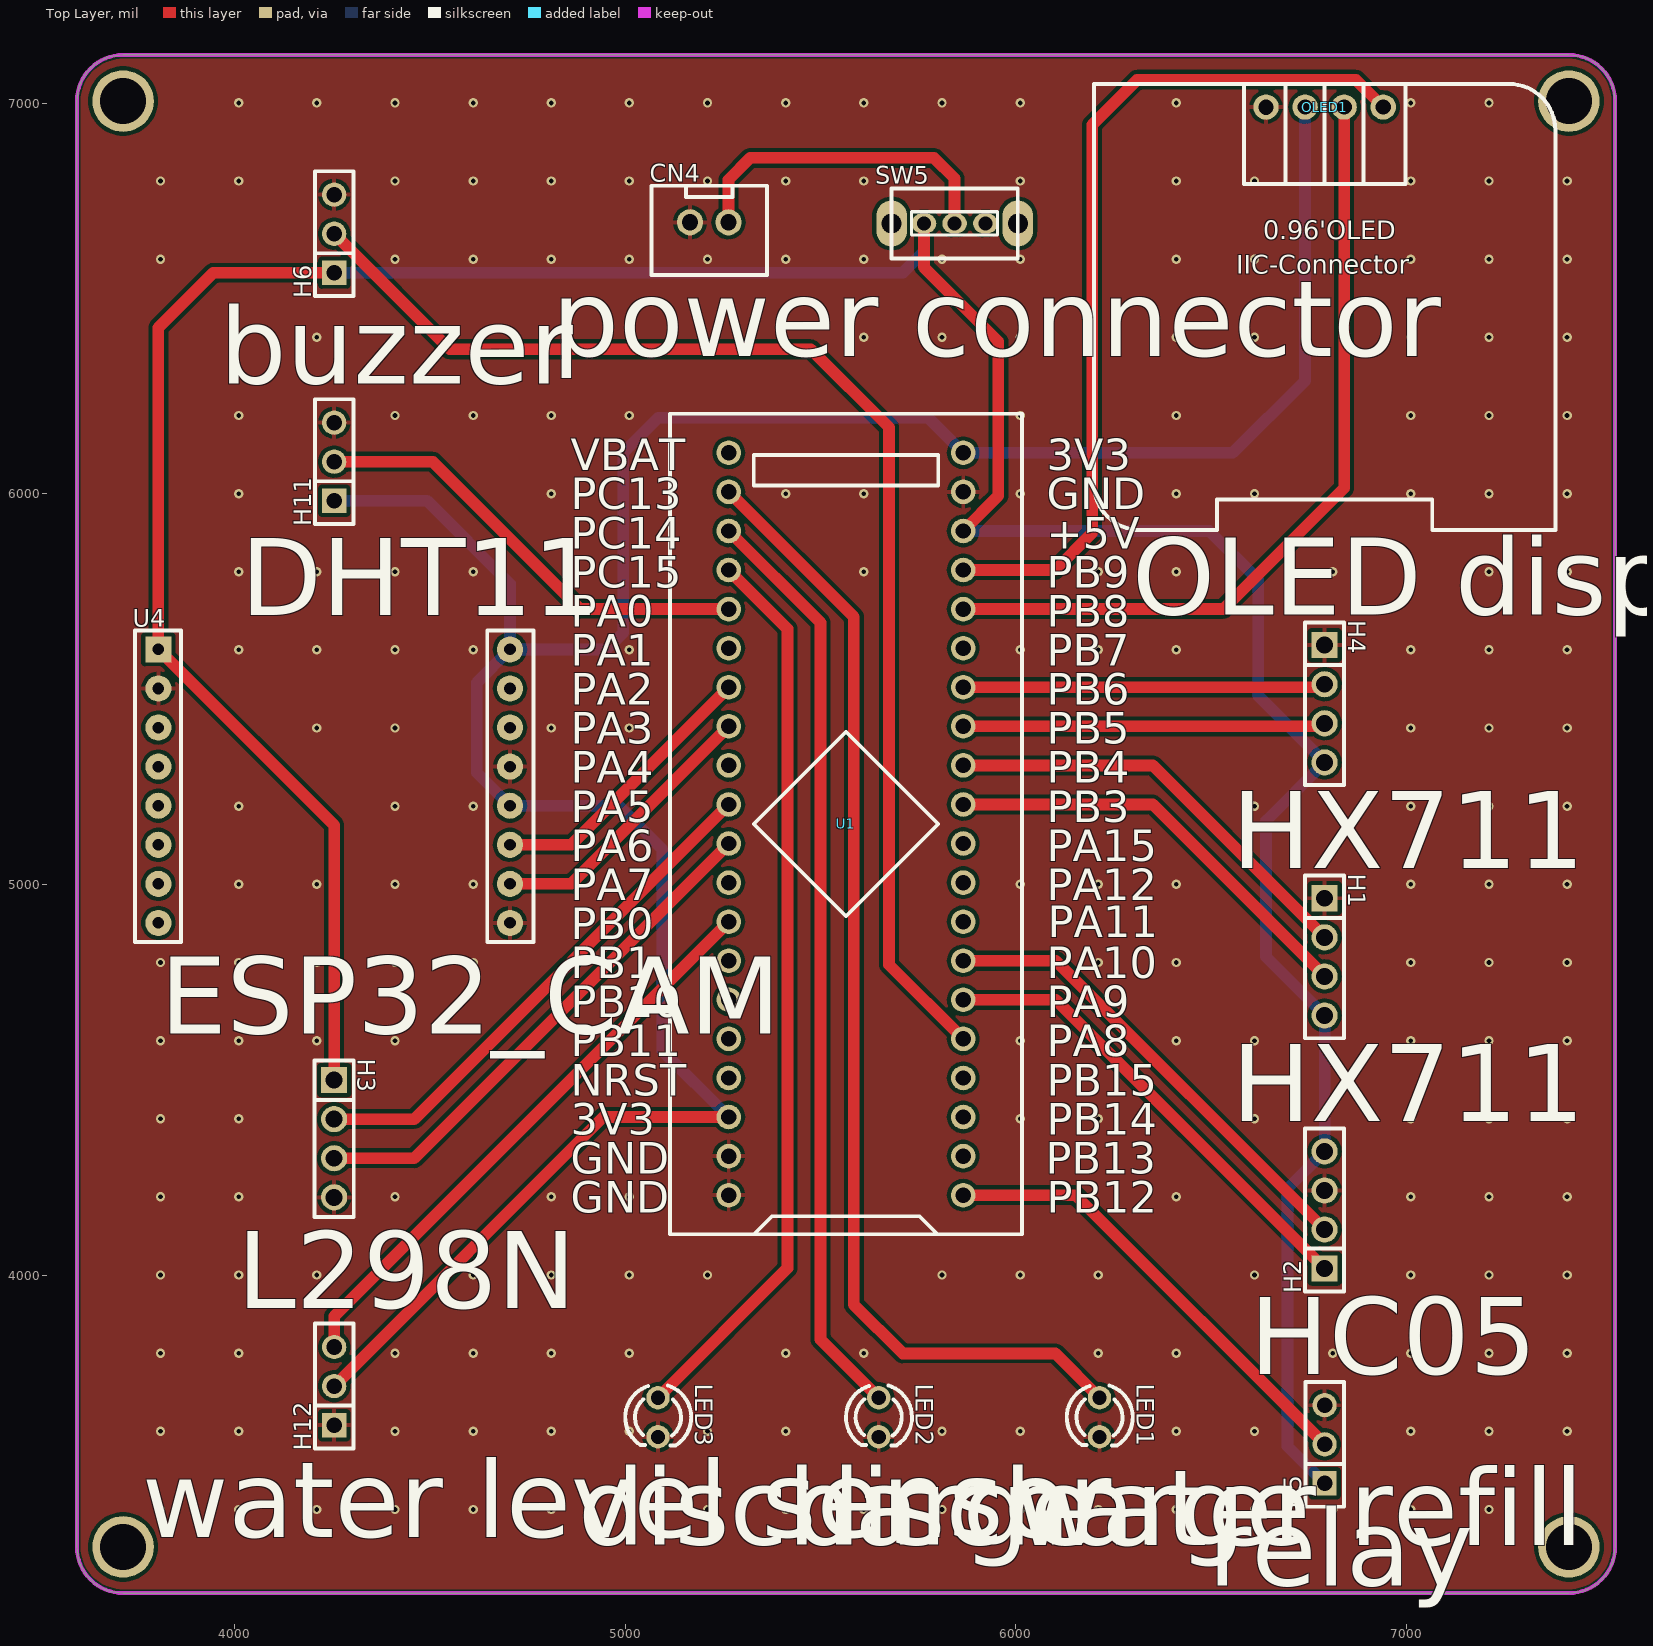
[diagram p0: Top Layer view]
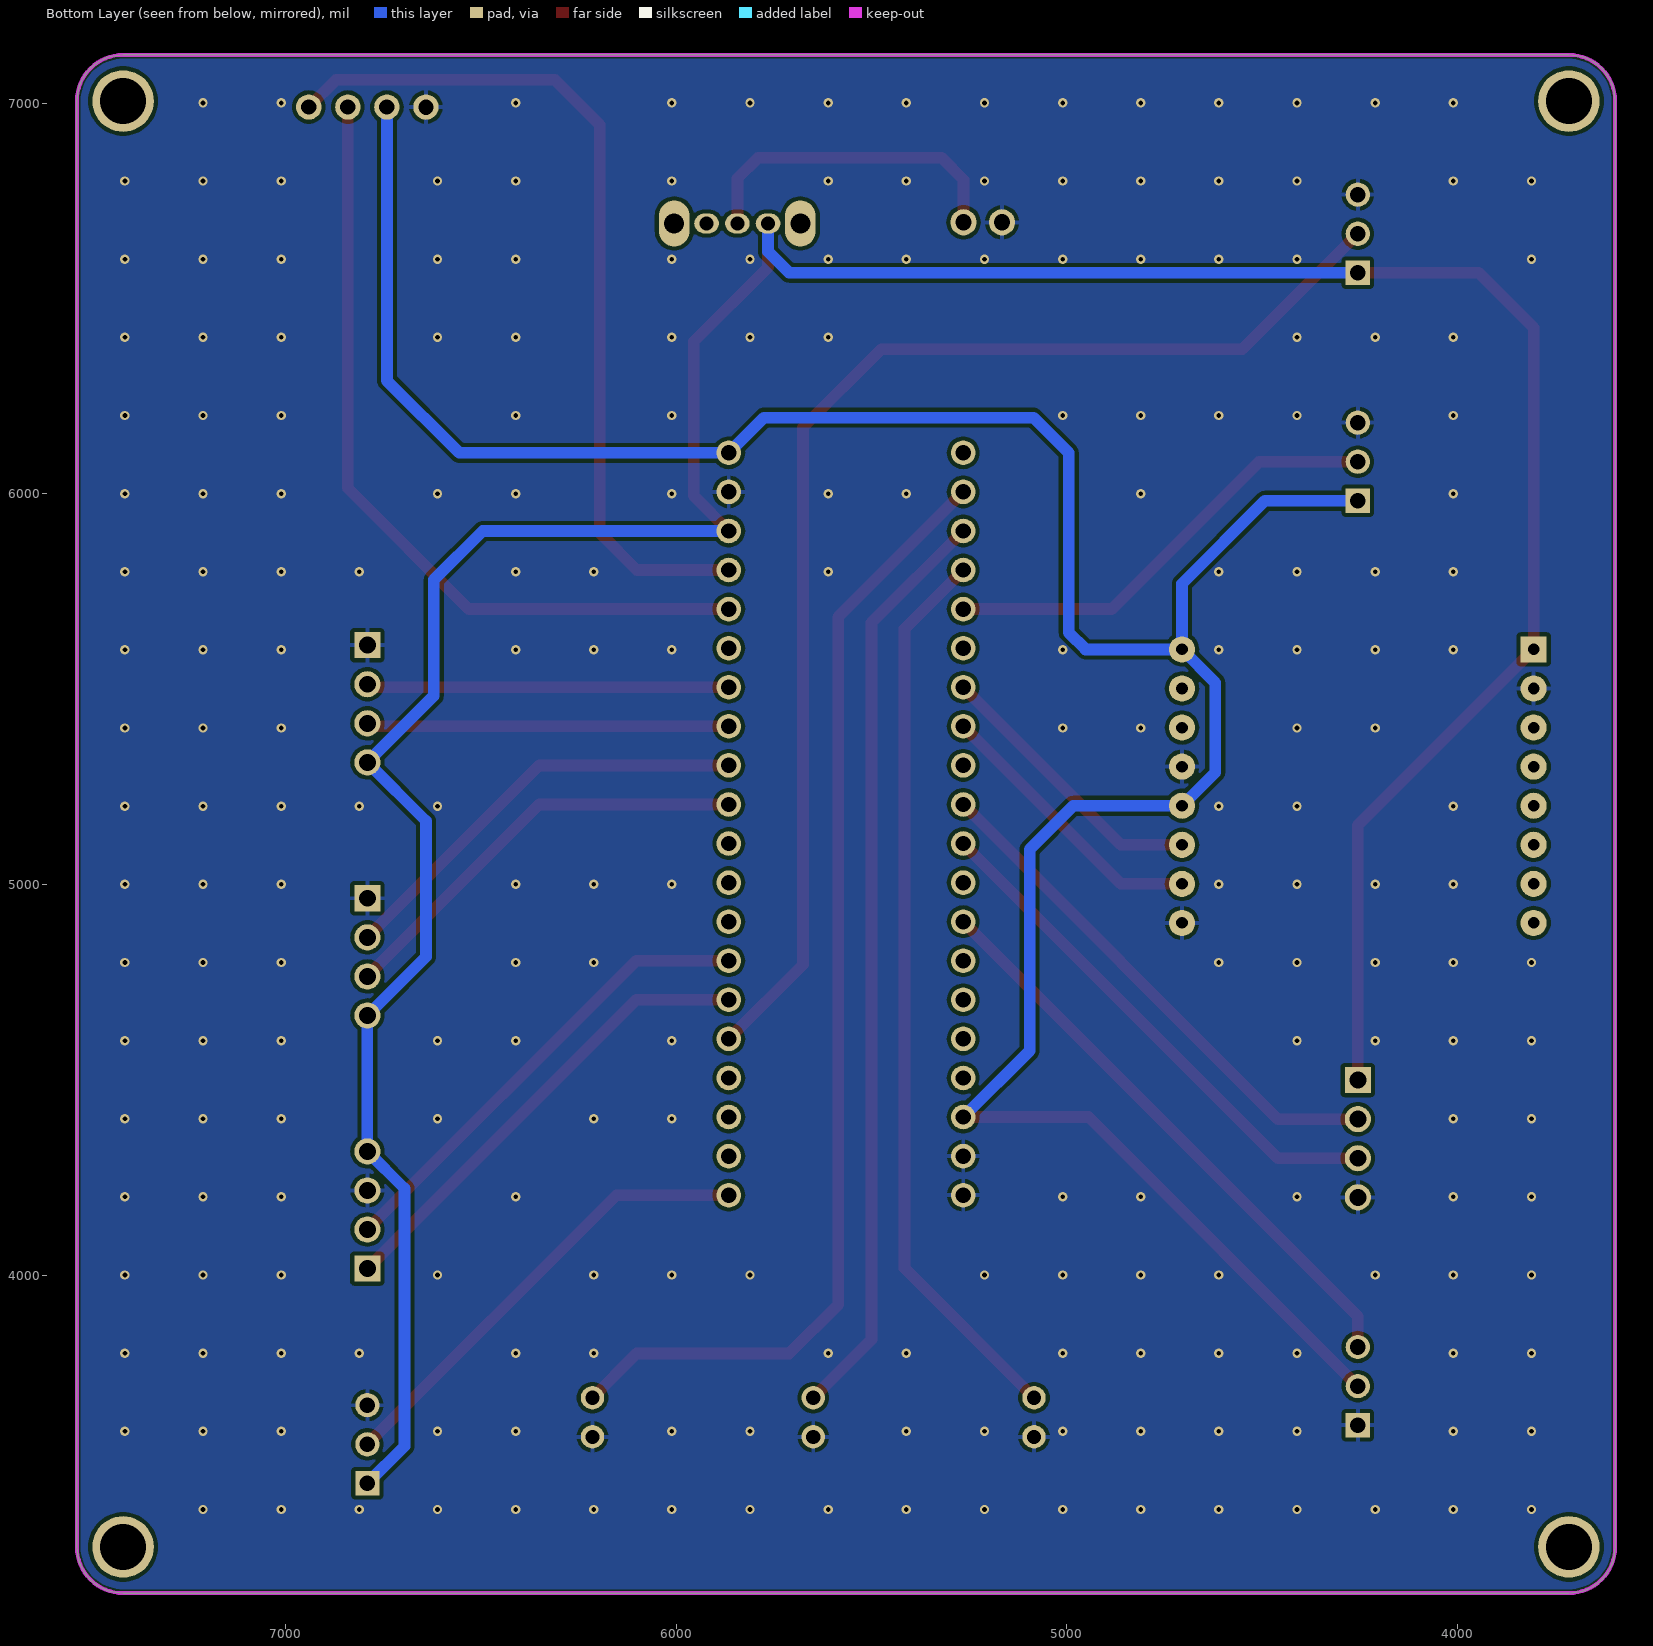
[diagram p1: Bottom Layer view, seen from below]
# Altium PCB MISC52091.pcbdoc
Units mil, origin at the board's own origin, x right, y up, seen from the top; angles counter-clockwise.
Board outline 3937.01 x 3937.01 mil, 2 copper layers (Top Layer, Bottom Layer), stack 62.206 mil thick; 16 components, 46 nets, 105 pads, 220 vias.

## Layer stack, top to bottom
Top Solder Mask Layer: solder mask 0.394, Dk 3.3
Top Layer: signal copper 1.379
Dielectric1: surface 59.449, FR4, Dk 4.5
Bottom Layer: signal copper 1.378
Bottom Solder Mask Layer: solder mask 0.394, Dk 3.3

## Board outline
3714.61,7123.5 ccw(c3714.61,7005.39) 3596.5,7005.39 3596.5,3304.61 ccw(c3714.61,3304.61) 3714.61,3186.5 7415.39,3186.5 ccw(c7415.39,3304.61) 7533.5,3304.61 7533.5,7005.39 ccw(c7415.39,7005.39) 7415.39,7123.5 3714.61,7123.5

## Design rules (kind name [scope] priority, off if disabled: settings)
BoardOutlineClearance copperThickness2oz_1 [All] p2 off: genericclearance=7.99 ignorepadtopadclearanceinfootprint=FALSE except(0: Arc-SplitContinuation Track-SplitContinuation SMDPad-SplitContinuation THPad-SplitContinuation Via-SplitContinuation Fill-SplitContinuation Region-SplitContinuation Poly-SplitContinuation Text-SplitContinuation Hole-SplitContinuation; 5.98: Arc-CutoutEdge Track-CutoutEdge SMDPad-CutoutEdge THPad-CutoutEdge Via-CutoutEdge Text-CutoutEdge; 6.9: Hole-OutlineEdge Hole-CutoutEdge; 10: Poly-OutlineEdge Poly-CutoutEdge; 11.81: Arc-OutlineEdge Track-OutlineEdge SMDPad-OutlineEdge THPad-OutlineEdge Via-OutlineEdge Fill-OutlineEdge Region-OutlineEdge Text-OutlineEdge Fill-CutoutEdge Region-CutoutEdge)
BoardOutlineClearance Plane_innerPlane_1 [All] p4 off: genericclearance=4.02 ignorepadtopadclearanceinfootprint=FALSE except(0: Arc-SplitContinuation Track-SplitContinuation SMDPad-SplitContinuation THPad-SplitContinuation Via-SplitContinuation Fill-SplitContinuation Region-SplitContinuation Poly-SplitContinuation Text-SplitContinuation Hole-SplitContinuation; 5.98: Arc-CutoutEdge Track-CutoutEdge SMDPad-CutoutEdge THPad-CutoutEdge Via-CutoutEdge Text-CutoutEdge; 6.9: Hole-OutlineEdge Hole-CutoutEdge; 10: Poly-OutlineEdge Poly-CutoutEdge; 11.81: Arc-OutlineEdge Track-OutlineEdge SMDPad-OutlineEdge THPad-OutlineEdge Via-OutlineEdge Fill-OutlineEdge Region-OutlineEdge Text-OutlineEdge Fill-CutoutEdge Region-CutoutEdge)
BoardOutlineClearance Copper_copperRegion_1 [All] p6 off: genericclearance=4.02 ignorepadtopadclearanceinfootprint=FALSE except(0: Arc-SplitContinuation Track-SplitContinuation SMDPad-SplitContinuation THPad-SplitContinuation Via-SplitContinuation Fill-SplitContinuation Region-SplitContinuation Poly-SplitContinuation Text-SplitContinuation Hole-SplitContinuation; 5.98: Arc-CutoutEdge Track-CutoutEdge SMDPad-CutoutEdge THPad-CutoutEdge Via-CutoutEdge Text-CutoutEdge; 6.9: Hole-OutlineEdge Hole-CutoutEdge; 10: Poly-OutlineEdge Poly-CutoutEdge; 11.81: Arc-OutlineEdge Track-OutlineEdge SMDPad-OutlineEdge THPad-OutlineEdge Via-OutlineEdge Fill-OutlineEdge Region-OutlineEdge Text-OutlineEdge Fill-CutoutEdge Region-CutoutEdge)
BoardOutlineClearance copperThickness1oz_1 [All] p8: genericclearance=4.02 ignorepadtopadclearanceinfootprint=FALSE except(0: Arc-SplitContinuation Track-SplitContinuation SMDPad-SplitContinuation THPad-SplitContinuation Via-SplitContinuation Fill-SplitContinuation Region-SplitContinuation Poly-SplitContinuation Text-SplitContinuation Hole-SplitContinuation; 5.98: Arc-CutoutEdge Track-CutoutEdge SMDPad-CutoutEdge THPad-CutoutEdge Via-CutoutEdge Text-CutoutEdge; 6.9: Hole-OutlineEdge Hole-CutoutEdge; 10: Poly-OutlineEdge Poly-CutoutEdge; 11.81: Arc-OutlineEdge Track-OutlineEdge SMDPad-OutlineEdge THPad-OutlineEdge Via-OutlineEdge Fill-OutlineEdge Region-OutlineEdge Text-OutlineEdge Fill-CutoutEdge Region-CutoutEdge)
Clearance copperThickness2oz [All] p1 off: gap=7.99 ignorepadtopadclearanceinfootprint=FALSE except(5.98: SMDPad-Track SMDPad-SMDPad THPad-Track SMDPad-THPad THPad-THPad Track-Via SMDPad-Via THPad-Via Via-Via Fill-SMDPad Region-SMDPad Fill-THPad Region-THPad Fill-Via Region-Via Fill-Fill Fill-Region Region-Region Arc-Track Arc-SMDPad Arc-THPad Arc-Via Fill-Arc Region-Arc Arc-Arc Text-Track SMDPad-Text Text-THPad Text-Via Fill-Text Region-Text Arc-Text Text-Text; 6.9: Hole-Track Hole-SMDPad Hole-THPad Hole-Via Fill-Hole Region-Hole Hole-Arc Hole-Text; 10: Poly-Track Poly-SMDPad Poly-THPad Poly-Via Poly-Fill Poly-Region Poly-Poly Poly-Arc Poly-Text Poly-Hole; 11.81: Fill-Track Region-Track)
Clearance Plane_innerPlane [All] p3 off: gap=4.02 ignorepadtopadclearanceinfootprint=FALSE except(5.98: SMDPad-Track SMDPad-SMDPad THPad-Track SMDPad-THPad THPad-THPad Track-Via SMDPad-Via THPad-Via Via-Via Fill-SMDPad Region-SMDPad Fill-THPad Region-THPad Fill-Via Region-Via Fill-Fill Fill-Region Region-Region Arc-Track Arc-SMDPad Arc-THPad Arc-Via Fill-Arc Region-Arc Arc-Arc Text-Track SMDPad-Text Text-THPad Text-Via Fill-Text Region-Text Arc-Text Text-Text; 6.9: Hole-Track Hole-SMDPad Hole-THPad Hole-Via Fill-Hole Region-Hole Hole-Arc Hole-Text; 10: Poly-Track Poly-SMDPad Poly-THPad Poly-Via Poly-Fill Poly-Region Poly-Poly Poly-Arc Poly-Text Poly-Hole; 11.81: Fill-Track Region-Track)
Clearance Copper_copperRegion [All] p5 off: gap=4.02 ignorepadtopadclearanceinfootprint=FALSE except(5.98: SMDPad-Track SMDPad-SMDPad THPad-Track SMDPad-THPad THPad-THPad Track-Via SMDPad-Via THPad-Via Via-Via Fill-SMDPad Region-SMDPad Fill-THPad Region-THPad Fill-Via Region-Via Fill-Fill Fill-Region Region-Region Arc-Track Arc-SMDPad Arc-THPad Arc-Via Fill-Arc Region-Arc Arc-Arc Text-Track SMDPad-Text Text-THPad Text-Via Fill-Text Region-Text Arc-Text Text-Text; 6.9: Hole-Track Hole-SMDPad Hole-THPad Hole-Via Fill-Hole Region-Hole Hole-Arc Hole-Text; 10: Poly-Track Poly-SMDPad Poly-THPad Poly-Via Poly-Fill Poly-Region Poly-Poly Poly-Arc Poly-Text Poly-Hole; 11.81: Fill-Track Region-Track)
Clearance copperThickness1oz [All] p7: gap=4.02 ignorepadtopadclearanceinfootprint=FALSE except(5.98: SMDPad-Track SMDPad-SMDPad THPad-Track SMDPad-THPad THPad-THPad Track-Via SMDPad-Via THPad-Via Via-Via Fill-SMDPad Region-SMDPad Fill-THPad Region-THPad Fill-Via Region-Via Fill-Fill Fill-Region Region-Region Arc-Track Arc-SMDPad Arc-THPad Arc-Via Fill-Arc Region-Arc Arc-Arc Text-Track SMDPad-Text Text-THPad Text-Via Fill-Text Region-Text Arc-Text Text-Text; 6.9: Hole-Track Hole-SMDPad Hole-THPad Hole-Via Fill-Hole Region-Hole Hole-Arc Hole-Text; 10: Poly-Track Poly-SMDPad Poly-THPad Poly-Via Poly-Fill Poly-Region Poly-Poly Poly-Arc Poly-Text Poly-Hole; 11.81: Fill-Track Region-Track)
DiffPairsRouting differentialPair [All] p1: maxlimit=6 minlimit=6 mostfreqgap=6 toplayer_minwidth=5 toplayer_prefwidth=10 toplayer_maxwidth=100 toplayer_mingap=6 toplayer_prefgap=6 toplayer_maxgap=6 bottomlayer_minwidth=5 bottomlayer_prefwidth=10 bottomlayer_maxwidth=100 bottomlayer_mingap=6 bottomlayer_prefgap=6 bottomlayer_maxgap=6 maxuncoupledlength=10
HoleToHoleClearance otherClearance [All] p1: gap=11.81 allowstackedmicrovias=TRUE
Length netLength [All] p1: minlimit=0 maxlimit=0
PasteMaskExpansion pasteMaskExpansion [All] p1: expansion=0
PlaneConnect innerPlane [All] p1: planeconnectstyle=Relief reliefexpansion=20 reliefentries=4 reliefconductorwidth=10 reliefairgap=10
PolygonConnect copperRegion [All] p1: connectstyle=Relief reliefconductorwidth=10 reliefentries=4 polygonreliefangle="90 Angle" airgapwidth=10 via.connectstyle=Relief via.reliefconductorwidth=10 via.reliefentries=4 via.polygonreliefangle="90 Angle" via.airgapwidth=10
RoutingVias viaSize [All] p1: holewidth=12.01 width=24.02 viastyle="Through Hole" minholewidth=11.81 minwidth=19.68 maxholewidth=248.03 maxwidth=393.7
SolderMaskExpansion solderMaskExpansion [IsVia] p1: expansion=-1000 istentingtop=TRUE
SolderMaskExpansion solderMaskExpansion [All] p2: expansion=2 istentingtop=FALSE
Width copperThickness2oz_2 [All] p1 off: maxlimit=100 minlimit=8 preferedwidth=10
Width copperThickness1oz_2 [All] p2: maxlimit=100 minlimit=5 preferedwidth=10

## Components (designator, comment, footprint, x,y, rotation, side; value= is the part's Value field where it differs from the comment)
CN4 "XH2.54*2P_through-hole" CONN-TH_2P-P2.50-XH2.54-2P 5215,6695 r0 top
H1 "" HDR-TH_4P-P2.54-V-F 6790,4814.92 r270 top
H2 "" HDR-TH_4P-P2.54-V-F 6790,4167.11 r90 top
H3 "" HDR-TH_4P-P2.54-V-M 4255,4349.55 r270 top
H4 "" HDR-TH_4P-P2.54-V-F 6790,5462.74 r270 top
H5 "" HDR-TH_3P-P2.54-V-F 6790,3567.42 r90 top
H6 "" HDR-TH_3P-P2.54-V-F 4255,6665.74 r90 top
H11 "" HDR-TH_3P-P2.54-V-F 4255,6082.21 r90 top
H12 "" HDR-TH_3P-P2.54-V-F 4255,3716.31 r90 top
LED1 "" LED_TH-3mm 6213.82,3636.52 r270 top
LED2 "" LED_TH-3mm 5648.82,3636.52 r270 top
LED3 "" LED_TH-3mm 5083.82,3636.52 r270 top
OLED1 "" 0.96OLED_4P 6790,6990 r0 top
SW5 "" 拨动开关 5837.9,6692.05 r0 top
U1 "STM32F103C8T6-Card" CONN-TH_L53.3-W22.9_STM32F103C8T6-CARD 5565,5155 r90 top
U4 "ESP32_CAM" ESP32-CAM 4255,5251.76 r0 top

## Footprints (in the part's own frame and the unit in brackets; to place one, negate y for a bottom-side part, rotate by r counter-clockwise, add the part's x,y. Pads: shape width x height; smd on the part's side, far side on the other; paste and mask are expansions set on the pad)
0.96OLED_4P [mm]
  round 1.65 hole 1 copper offset 0,0: 1(-3.81,-0.001) 2(-1.27,0.002) 3(1.27,0.002) 4(3.81,0.002)
  silkscreen extent -15,-27.5 15,1.5
CONN-TH_2P-P2.50-XH2.54-2P [mm]
  round 1.7 hole 1.05 paste+0 mask+0.05: 1(1.25,0) 2(-1.25,0)
  silkscreen extent -3.75,-3.42 3.75,2.37
CONN-TH_L53.3-W22.9_STM32F103C8T6-CARD [mm]
  round 1.6 hole 1: 1(-24.13,-7.62) 2(-21.59,-7.62) 3(-19.05,-7.62) 4(-16.51,-7.62) 5(-13.97,-7.62) 6(-11.43,-7.62) 7(-8.89,-7.62) 8(-6.35,-7.62) 9(-3.81,-7.62) 10(-1.27,-7.62) 11(1.27,-7.62) 12(3.81,-7.62) 13(6.35,-7.62) 14(8.89,-7.62) 15(11.43,-7.62) 16(13.97,-7.62) 17(16.51,-7.62) 18(19.05,-7.62) 19(21.59,-7.62) 20(24.13,-7.62) 21(24.13,7.62) 22(21.59,7.62) 23(19.05,7.62) 24(16.51,7.62) 25(13.97,7.62) 26(11.43,7.62) 27(8.89,7.62) 28(6.35,7.62) 29(3.81,7.62) 30(1.27,7.62) 31(-1.27,7.62) 32(-3.81,7.62) 33(-6.35,7.62) 34(-8.89,7.62) 35(-11.43,7.62) 36(-13.97,7.62) 37(-16.51,7.62) 38(-19.05,7.62) 39(-21.59,7.62) 40(-24.13,7.62)
  silkscreen extent -26.67,-11.43 26.67,11.43
ESP32-CAM [mm]
  rect 1.7x1.7 hole 0.75: 1(-11.43,8.89)
  round 1.7 hole 0.75: 2(-11.43,6.35) 3(-11.43,3.81) 4(-11.43,1.27) 5(-11.43,-1.27) 6(-11.43,-3.81) 7(-11.43,-6.35) 8(-11.43,-8.89) 9(11.43,-8.89) 10(11.43,-6.35) 11(11.43,-3.81) 12(11.43,-1.27) 13(11.43,1.27) 14(11.43,3.81) 15(11.43,6.35) 16(11.43,8.89)
  silkscreen extent -12.95,-10.13 12.95,10.13
HDR-TH_3P-P2.54-V-F [mil]
  rect 62x62 hole 40.16: 1(-100,0)
  round 62 hole 40.16: 2(0,0) 3(100,0)
  silkscreen extent -160,-49 160,49
HDR-TH_4P-P2.54-V-F [mm]
  rect 1.7x1.7 hole 1.1: 1(-3.81,0)
  round 1.7 hole 1.1: 2(-1.27,0) 3(1.27,0) 4(3.81,0)
  silkscreen extent -5.29,-1.27 5.29,1.27
HDR-TH_4P-P2.54-V-M [mm]
  rect 1.7x1.7 hole 1.1: 1(-3.81,0)
  round 1.7 hole 1.1: 2(-1.27,0) 3(1.27,0) 4(3.81,0)
  silkscreen extent -5.08,-1.27 5.08,1.27
LED_TH-3mm [mil]
  round 60 hole 36 paste+0 mask+2: 1(-50,0) 2(50,0)
  silkscreen extent -81,-84 72,85
拨动开关 [mil]
  oval 63x51.2 hole 35.4 paste+0 mask+2: 1(-73.4,0) 2(5,0) 3(84,0)
  oval 78.7x118.1 hole 51.2 paste+0 mask+2: 4(166.7,0) 5(-156.1,0)
  silkscreen extent -156,-90 167,90

## Free pads (board coordinates)
  round 157.48 hole 118.11: 1(3714.61,7005.39) 1(3714.61,3304.61) 1(7415.39,7005.39) 1(7415.39,3304.61)

## Via types
v1: diameter 24.02, hole 12, Top Layer to Bottom Layer, 220 vias

## Nets (pads, with @x,y where several pads share a name; then routed paths per layer and width w, separated by ;. In a path a pad name is that pad's centre, name@x,y a point inside that pad or via, vN(x,y) a via of type N, cw(c..) or ccw(c..) an arc to the next point about the centre after c; other vN are vias at no path point)
$1N17171: CN4.1 SW5.2 | length 848
  Top Layer w30: CN4.1 5264.22,6804.22 5320,6860 5790,6860 5842.9,6807.1 SW5.2
+5V: H1.4 H2.4 H3.1 H4.4 H5.1 H6.1 SW5.1 U1.18 U4.1 | length 8520.4
  Top Layer w30: H3.1 4255,5151.76 U4.1 3805,6425 3945.74,6565.74 H6.1 ; SW5.1 5764.5,6580.5 5955,6390 5955,5995 U1.18
  Bottom Layer w30: H6.1 5710.74,6565.74 5764.5,6619.5 SW5.1 ; U1.18 6495,5905 6620,5780 6620,5482.73 H4.4 6640,5162.74 6640,4814.92 H1.4 H2.4 6695,4222.11 6695,3562.42 H5.1
GND: CN4.2 H1.1 H2.3 H3.4 H4.1 H5.3 H6.3 H11.3 H12.1 LED1.2 LED2.2 LED3.2 OLED1.1 U1.19 U1.39 U1.40 U4.2 U4.9 U4.13
  other v1: 3810.6,3400.6 4010.6,3400.6 4210.6,3400.6 4410.6,3400.6 4610.6,3400.6 4810.6,3400.6 5010.6,3400.6 5210.6,3400.6 5410.6,3400.6 5610.6,3400.6 5810.6,3400.6 6010.6,3400.6 6210.6,3400.6 6410.6,3400.6 6610.6,3400.6 6810.6,3400.6 7010.6,3400.6 7210.6,3400.6 3810.6,3600.6 4010.6,3600.6 4410.6,3600.6 4610.6,3600.6 4810.6,3600.6 5010.6,3600.6 5210.6,3600.6 5410.6,3600.6 5810.6,3600.6 6010.6,3600.6 6410.6,3600.6 6610.6,3600.6 7010.6,3600.6 7210.6,3600.6 7410.6,3600.6 3810.6,3800.6 4010.6,3800.6 4410.6,3800.6 4610.6,3800.6 4810.6,3800.6 5010.6,3800.6 5410.6,3800.6 5610.6,3800.6 6210.6,3800.6 6410.6,3800.6 6810.6,3800.6 7010.6,3800.6 7210.6,3800.6 7410.6,3800.6 3810.6,4000.6 4010.6,4000.6 4210.6,4000.6 4610.6,4000.6 4810.6,4000.6 5010.6,4000.6 5210.6,4000.6 5810.6,4000.6 6010.6,4000.6 6210.6,4000.6 6610.6,4000.6 7010.6,4000.6 7210.6,4000.6 7410.6,4000.6 3810.6,4200.6 4010.6,4200.6 4410.6,4200.6 4810.6,4200.6 5010.6,4200.6 6410.6,4200.6 7010.6,4200.6 7210.6,4200.6 7410.6,4200.6 3810.6,4400.6 4010.6,4400.6 6010.6,4400.6 6210.6,4400.6 6610.6,4400.6 7010.6,4400.6 7210.6,4400.6 7410.6,4400.6 3810.6,4600.6 4010.6,4600.6 4210.6,4600.6 4410.6,4600.6 6010.6,4600.6 6410.6,4600.6 6610.6,4600.6 7010.6,4600.6 7210.6,4600.6 7410.6,4600.6 3810.6,4800.6 4010.6,4800.6 4210.6,4800.6 4410.6,4800.6 4610.6,4800.6 6210.6,4800.6 6410.6,4800.6 7010.6,4800.6 7210.6,4800.6 7410.6,4800.6 4010.6,5000.6 4210.6,5000.6 4410.6,5000.6 4610.6,5000.6 6010.6,5000.6 6210.6,5000.6 6410.6,5000.6 7010.6,5000.6 7210.6,5000.6 7410.6,5000.6 4010.6,5200.6 4410.6,5200.6 4610.6,5200.6 6610.6,5200.6 6810.6,5200.6 7010.6,5200.6 7210.6,5200.6 7410.6,5200.6 4210.6,5400.6 4410.6,5400.6 4810.6,5400.6 5010.6,5400.6 7010.6,5400.6 7210.6,5400.6 7410.6,5400.6 4010.6,5600.6 4210.6,5600.6 4410.6,5600.6 4610.6,5600.6 5010.6,5600.6 6010.6,5600.6 6210.6,5600.6 6410.6,5600.6 7010.6,5600.6 7210.6,5600.6 7410.6,5600.6 4010.6,5800.6 4210.6,5800.6 4410.6,5800.6 4610.6,5800.6 5610.6,5800.6 6210.6,5800.6 6410.6,5800.6 6810.6,5800.6 7010.6,5800.6 7210.6,5800.6 7410.6,5800.6 4010.6,6000.6 4810.6,6000.6 5410.6,6000.6 5610.6,6000.6 6010.6,6000.6 6410.6,6000.6 6610.6,6000.6 7010.6,6000.6 7210.6,6000.6 7410.6,6000.6 4010.6,6200.6 4410.6,6200.6 4610.6,6200.6 4810.6,6200.6 5010.6,6200.6 6010.6,6200.6 6410.6,6200.6 7010.6,6200.6 7210.6,6200.6 7410.6,6200.6 4010.6,6400.6 4210.6,6400.6 4410.6,6400.6 5610.6,6400.6 5810.6,6400.6 6010.6,6400.6 6410.6,6400.6 6610.6,6400.6 7010.6,6400.6 7210.6,6400.6 7410.6,6400.6 3810.6,6600.6 4410.6,6600.6 4610.6,6600.6 4810.6,6600.6 5010.6,6600.6 5210.6,6600.6 5410.6,6600.6 5610.6,6600.6 5810.6,6600.6 6010.6,6600.6 6410.6,6600.6 6610.6,6600.6 7010.6,6600.6 7210.6,6600.6 7410.6,6600.6 3810.6,6800.6 4010.6,6800.6 4410.6,6800.6 4610.6,6800.6 4810.6,6800.6 5010.6,6800.6 5210.6,6800.6 5410.6,6800.6 5610.6,6800.6 6010.6,6800.6 6410.6,6800.6 6610.6,6800.6 7010.6,6800.6 7210.6,6800.6 7410.6,6800.6 4010.6,7000.6 4210.6,7000.6 4410.6,7000.6 4610.6,7000.6 4810.6,7000.6 5010.6,7000.6 5210.6,7000.6 5410.6,7000.6 5610.6,7000.6 5810.6,7000.6 6010.6,7000.6 6410.6,7000.6 7010.6,7000.6 7210.6,7000.6
IO0: U4.14
IO2: U4.7
IO4: U4.8
IO12: U4.3
IO13: U4.4
IO14: U4.6
IO15: U4.5
IO16: U4.15
NRST: U1.37
PA0: H11.2 U1.25 | length 1166.2
  Top Layer w30: H11.2 4507.79,6082.21 4885,5705 U1.25
PA1: U1.26
PA2: U1.27 U4.11 | length 727
  Top Layer w30: U4.11 4861.76,5101.76 U1.27
PA3: U1.28 U4.10 | length 727
  Top Layer w30: U4.10 4861.76,5001.76 U1.28
PA4: U1.29
PA5: H3.2 U1.30 | length 1343.6
  Top Layer w30: H3.2 4459.54,4399.55 U1.30
PA6: H3.3 U1.31 | length 1343.6
  Top Layer w30: H3.3 4459.54,4299.55 U1.31
PA7: U1.32
PA8: H6.2 U1.5 | length 3269
  Top Layer w30: H6.2 4550.74,6370 5475,6370 5675,6170 5675,4795 U1.5
PA9: H2.1 U1.6 | length 1209.9
  Top Layer w30: U1.6 6102.1,4705 H2.1
PA10: H2.2 U1.7 | length 1209.9
  Top Layer w30: U1.7 6102.1,4805 H2.2
PA11: U1.8
PA12: U1.9
PA15: U1.10
PB0: H12.3 U1.33 | length 1507
  Top Layer w30: H12.3 4255,3895 U1.33
PB1: U1.34
PB3: H1.3 U1.11 | length 1107.3
  Top Layer w30: U1.11 6349.92,5205 H1.3
PB4: H1.2 U1.12 | length 1107.3
  Top Layer w30: U1.12 6349.92,5305 H1.2
PB5: H4.3 U1.13 | length 928.2
  Top Layer w30: U1.13 6782.26,5405 H4.3
PB6: H4.2 U1.14 | length 928.2
  Top Layer w30: U1.14 6782.26,5505 H4.2
PB7: U1.15
PB8: OLED1.3 U1.16 | length 2078.5
  Top Layer w30: U1.16 6530,5705 6840,6015 OLED1.3@6840,6990.05
PB9: OLED1.4 U1.17 | length 2236
  Top Layer w30: U1.17 6100,5805 6195,5900 6195,6945 6310,7060 6870.05,7060 OLED1.4@6940,6990.05
PB10: U1.35
PB11: U1.36
PB12: H5.2 U1.1 | length 1189.1
  Top Layer w30: U1.1 6152.42,4205 H5.2
PB13: U1.2
PB14: U1.3
PB15: U1.4
PC13: LED1.1 U1.22 | length 2940.1
  Top Layer w30: U1.22 5585,5685 5585,3925 5710,3800 6100.33,3800 LED1.1
PC14: LED2.1 U1.23 | length 2377.5
  Top Layer w30: U1.23 5500,5670 5500,3835.33 LED2.1
PC15: LED3.1 U1.24 | length 2317.8
  Top Layer w30: LED3.1 5415,4017.7 5415,5655 U1.24
VBAT: U1.21
VCC: H11.1 H12.2 OLED1.2 U1.20 U1.38 U4.12 U4.16 | length 7027.7
  Top Layer w30: H12.2 4943.69,4405 U1.38
  Bottom Layer w30: H11.1 4492.79,5982.21 4705,5770 U4.16 ; U1.38 5095,4575 5095,5090 4983.24,5201.76 U4.12 4620,5286.76 4620,5516.76 U4.16 ; OLED1.2@6740,6990.05 6740,6290 6555,6105 U1.20 5775,6195 5085,6195 4995,6105 4995,5645 4951.76,5601.76 U4.16
pads on no net: SW5.3 SW5.4 SW5.5

## Polygon pours and split planes (outlines as drawn)
GND on Bottom Layer (solid, remove dead copper, pour order 2): 3525,7245 3525,3080 7700,3080 7700,7245
GND on Top Layer (solid, remove dead copper, pour order 2): 3000,7415 3000,3000 7930,3000 7930,7415

## Keep-outs
Board Outline Layer:
  the board outline again, w10

## Silkscreen, mask and mechanical layers (free items; w line width, h text height)
Top Silkscreen Layer:
  text "power connector" at 4812.87,6351.57 h196.85
  text "buzzer" at 3961.81,6282.11 h196.85
  text "VBAT" at 4860.95,6060 h80
  text "3V3" at 6079.16,6060 h80
  text "PC13" at 4860.95,5960 h80
  text "GND" at 6079.16,5960 h80
  text "PC14" at 4860.95,5860 h80
  text "+5V" at 6079.16,5860 h80
  text "PC15" at 4860.95,5760 h80
  text "PB9" at 6079.16,5760 h80
  text "OLED display" at 6298.02,5690.76 h196.85
  text "DHT11" at 4016.39,5689.33 h196.85
  text "PA0" at 4860.95,5660 h80
  text "PB8" at 6079.16,5660 h80
  text "PA1" at 4860.95,5560 h80
  text "PB7" at 6079.16,5560 h80
  text "PA2" at 4860.95,5460 h80
  text "PB6" at 6079.16,5460 h80
  text "PA3" at 4860.95,5360 h80
  text "PB5" at 6079.16,5360 h80
  text "PA4" at 4860.95,5260 h80
  text "PB4" at 6079.16,5260 h80
  text "PA5" at 4860.95,5160 h80
  text "PB3" at 6079.16,5160 h80
  text "PA6" at 4860.95,5060 h80
  text "PA15" at 6079.16,5060 h80
  text "HX711" at 6552.43,5042.34 h196.85
  text "PA7" at 4860.95,4960 h80
  text "PA12" at 6079.16,4960 h80
  text "PA11" at 6080.95,4865 h80
  text "PB0" at 4860.95,4860 h80
  text "PB1" at 4860.95,4760 h80
  text "PA10" at 6079.16,4760 h80
  text "PB10" at 4860.95,4660 h80
  text "PA9" at 6079.16,4660 h80
  text "ESP32_CAM" at 3810,4617.64 h196.85
  text "PB11" at 4860.95,4560 h80
  text "PA8" at 6079.16,4560 h80
  text "NRST" at 4860.95,4460 h80
  text "PB15" at 6079.16,4460 h80
  text "HX711" at 6552.43,4394.53 h196.85
  text "3V3" at 4860.95,4360 h80
  text "PB14" at 6079.16,4360 h80
  text "GND" at 4860.95,4260 h80
  text "PB13" at 6075.95,4260 h80
  text "GND" at 4860.95,4160 h80
  text "PB12" at 6079.16,4160 h80
  text "L298N" at 4007,3916.22 h196.85
  text "HC05" at 6597.92,3746.42 h196.85
  text "water level sensor" at 3763.77,3330 h196.85
  text "discharge" at 4880,3310 h196.85
  text "discharge" at 5433.11,3310 h196.85
  text "water refill" at 5998.15,3309.11 h196.85
  text "relay" at 6492.48,3205 h196.85